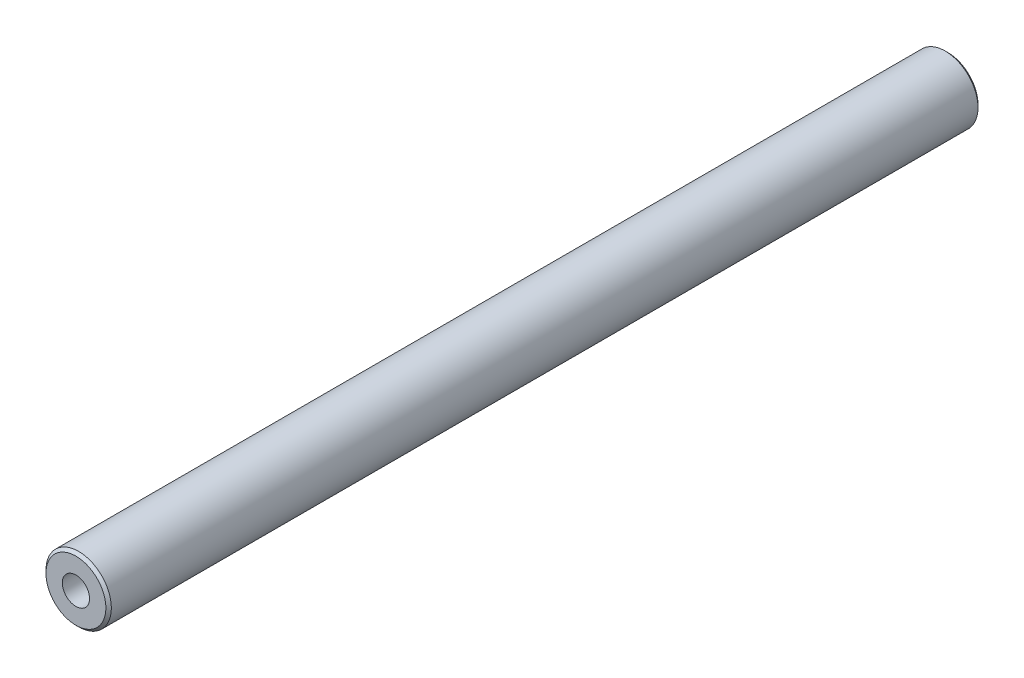
SolidWorks part; units mm, degrees
ref_plane "Front Plane" through (0, 0, 0) normal (0, 0, 1) x (1, 0, 0)
ref_plane "Top Plane" through (0, 0, 0) normal (0, 1, 0) x (1, 0, 0)
ref_plane "Right Plane" through (0, 0, 0) normal (1, 0, 0) x (0, 0, -1)
sketch "Sketch1" plane through (0, 0, 0) normal (0, 0, 1) x (1, 0, 0)
  circle A0 centre (0, 0) radius 6
  dimension "D1" = 12
extrude "Boss-Extrude1" add sketch "Sketch1" along normal blind 160
hole_wizard "M6 Tapped Hole1" positions "Sketch3" profile "Sketch2" tap size "M6" standard "GB"
sketch "Sketch3" plane through (0, 0, 160) normal (0, 0, 1) x (1, 0, 0)
  point P0 (0, 0)
sketch "Sketch2" plane through (0, 0, 160) normal (1, 0, 0) x (0, -1, 0)
  line L0 (0, 0) -> (0, 16.5022)
  line L1 (0, 16.5022) -> (2.5, 15)
  line L2 (2.5, 15) -> (2.5, 0)
  line L5 (2.5, 0) -> (0, 0)
  line L10 (0, 16.5022) -> (-2.5, 15) construction
  line L11 (0, -6.35) -> (0, 107.95) construction
  dimension "螺纹孔钻头直径" = 5
  dimension "螺纹孔钻头深度" = 15
  dimension "导头角度" = 118
cosmetic thread "Cosmetic Thread1" parameters "D1"=12, "D2"=6
chamfer "Chamfer1" distance 0.5 angle 45 2 edges at (6, 0, 0) (6, 0, 160)
